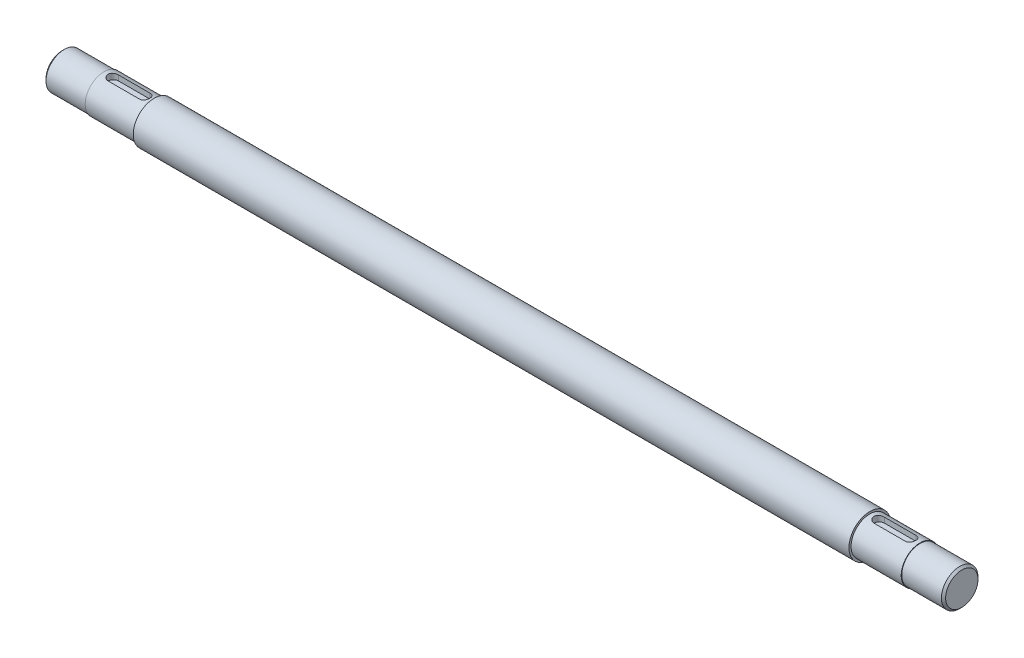
SolidWorks part; units mm, degrees
ref_plane "前视基准面" through (0, 0, 0) normal (0, 0, 1) x (1, 0, 0)
ref_plane "上视基准面" through (0, 0, 0) normal (0, 1, 0) x (1, 0, 0)
ref_plane "右视基准面" through (0, 0, 0) normal (1, 0, 0) x (0, 0, -1)
sketch "草图1" plane through (0, 0, 0) normal (1, 0, 0) x (0, 0, -1)
  circle A0 centre (0, 0) radius 20
extrude "凸台-拉伸1" add sketch "草图1" along normal mid plane 685
sketch "草图2" plane through (-342.5, 0, 0) normal (-1, 0, 0) x (0, 0, 1)
  circle A0 centre (0, 0) radius 18
extrude "凸台-拉伸2" add sketch "草图2" along normal blind 48
sketch "草图3" plane through (-390.5, 0, 0) normal (-1, 0, 0) x (0, 0, 1)
  circle A0 centre (0, 0) radius 17.5
extrude "凸台-拉伸3" add sketch "草图3" along normal blind 40
sketch "草图4" plane through (342.5, 0, 0) normal (1, 0, 0) x (0, 0, -1)
  circle A0 centre (0, 0) radius 18
extrude "凸台-拉伸4" add sketch "草图4" along normal blind 48
sketch "草图5" plane through (390.5, 0, 0) normal (1, 0, 0) x (0, 0, -1)
  circle A0 centre (0, 0) radius 17.5
extrude "凸台-拉伸5" add sketch "草图5" along normal blind 40
ref_plane "基准面1" through (0, 18, 0) normal (0, 1, 0) x (1, 0, 0)
sketch "草图7" plane through (0, 18, 0) normal (0, 1, 0) x (1, 0, 0)
  line L0 (351.5, 0) -> (381.5, 0) construction
  line L1 (342.5, -20) -> (342.5, 20) construction
  line L2 (351.5, 5) -> (381.5, 5)
  line L3 (351.5, -5) -> (381.5, -5)
  line L4 (-351.5, 0) -> (-381.5, 0) construction
  line L6 (-351.5, -5) -> (-381.5, -5)
  line L7 (-351.5, 5) -> (-381.5, 5)
  line L8 (-342.5, 18) -> (-342.5, -18) construction
  arc A0 (351.5, 5) -> (351.5, -5) centre (351.5, 0) ccw
  arc A1 (381.5, -5) -> (381.5, 5) centre (381.5, 0) ccw
  arc A2 (-351.5, -5) -> (-351.5, 5) centre (-351.5, 0) ccw
  arc A3 (-381.5, 5) -> (-381.5, -5) centre (-381.5, 0) ccw
  point P5 (366.5, 0)
  point P14 (-366.5, 0)
  dimension "D1" = 30
  dimension "D2" = 5
  dimension "D3" = 9
  dimension "D5" = 5
  dimension "D6" = 9
  dimension "D4" = 30
extrude "切除-拉伸1" cut sketch "草图7" against normal blind 5.71
chamfer "倒角1" distance 2 angle 45 2 edges at (-430.5, 0, 17.5) (430.5, 0, -17.5)
